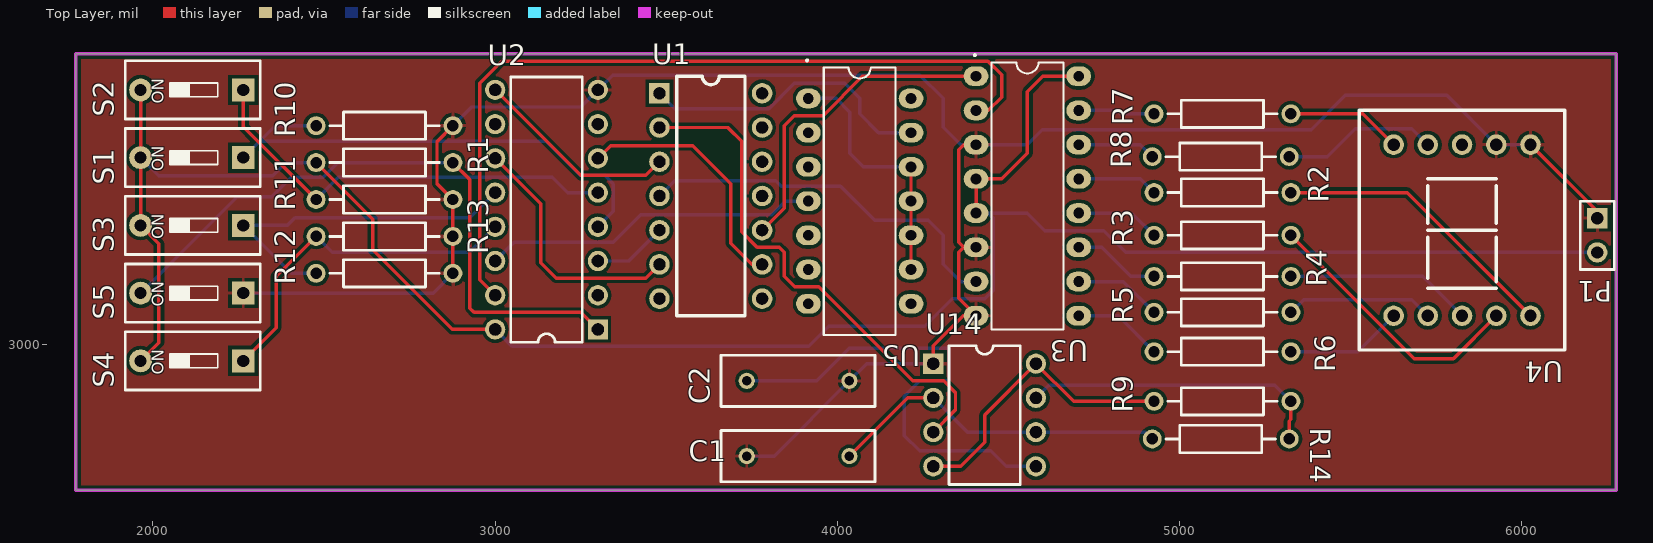
[diagram p0: Top Layer view]
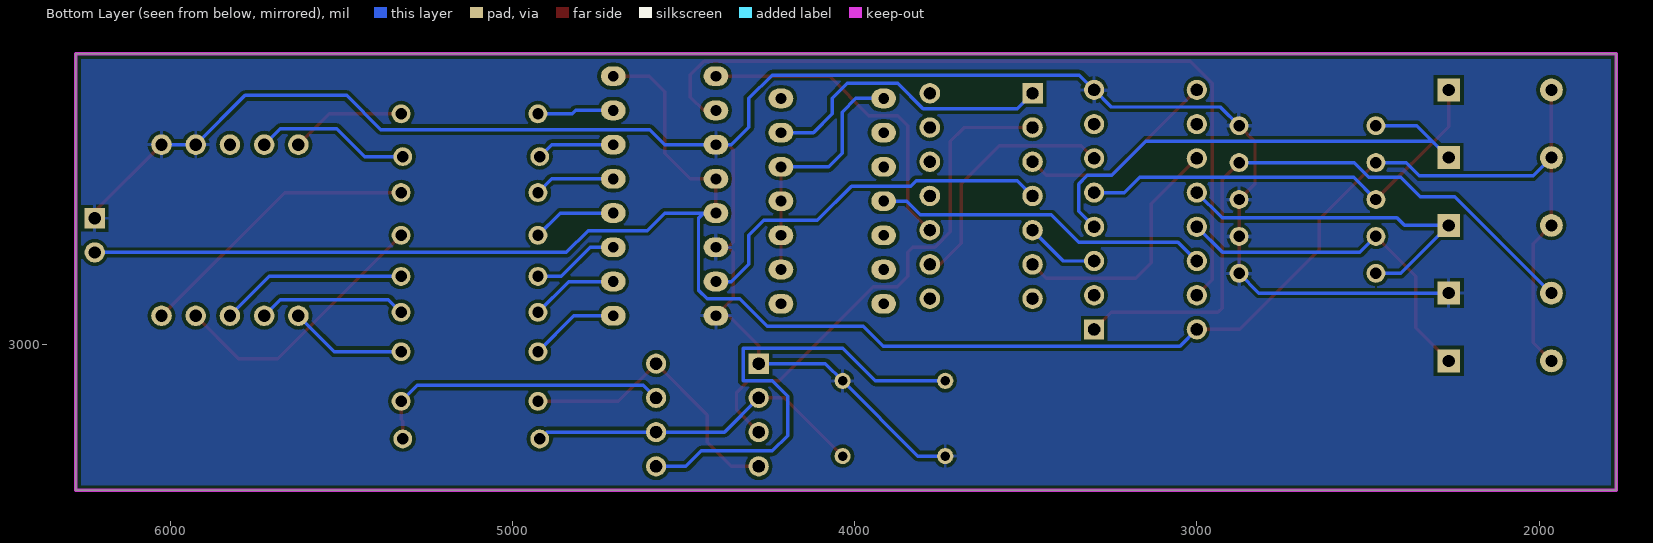
[diagram p1: Bottom Layer view, seen from below]
# Altium PCB MISC80628.PcbDoc
Units mil, origin at the board's own origin, x right, y up, seen from the top; angles counter-clockwise.
Board outline 4500 x 1275 mil, 2 copper layers (Top Layer, Bottom Layer); 28 components, 36 nets, 122 pads, 0 vias.

## Layer stack, top to bottom (the 12.6 mil dielectric is the usual default, probably not edited)
Top Solder: solder mask 0.4, Solder Resist, Dk 3.5
Top Layer: signal copper 1.4
Dielectric 1: dielectric 12.6, FR-4, Dk 4.8
Bottom Layer: signal copper 1.4
Bottom Solder: solder mask 0.4, Solder Resist, Dk 3.5

## Board outline
1775,2575 1775,3850 6275,3850 6275,2575

## Design rules (kind name [scope] priority, off if disabled: settings)
Clearance [All] p1: gap=10
PolygonConnect [All] p1: connectstyle=Relief reliefconductorwidth=10 reliefentries=4 polygonreliefangle="90 Angle" airgapwidth=10
RoutingVias [All] p1: holewidth=28 width=50 viastyle="Through Hole" minholewidth=28 minwidth=50 maxholewidth=28 maxwidth=50
SolderMaskExpansion [All] p1: expansion=4
Width [All] p1: maxlimit=10 minlimit=10 preferedwidth=10
30 further rules are at their usual default settings.

## Components (designator, comment, footprint, x,y, rotation, side; value= is the part's Value field where it differs from the comment)
C1 "Cap" RAD-0.3 3885,2675 r0 top
C2 "Cap" RAD-0.3 3885,2895 r180 top
P1 "Header 2" HDR1X2 6220,3370 r270 top
R1 "Res2" AXIAL-0.4 2676.56,3532.56 r180 top
R2 "Res2" AXIAL-0.4 5125,3445 r180 top
R3 "Res2" AXIAL-0.4 5125,3320 r180 top
R4 "Res2" AXIAL-0.4 5125,3200 r180 top
R5 "Res2" AXIAL-0.4 5125,3095 r180 top
R6 "Res2" AXIAL-0.4 5125,2980 r180 top
R7 "Res2" AXIAL-0.4 5125,3675 r180 top
R8 "Res2" AXIAL-0.4 5120,3550 r180 top
R9 "Res2" AXIAL-0.4 5125,2835 r180 top
R10 "Res2" AXIAL-0.4 2676.56,3640.43 r180 top
R11 "Res2" AXIAL-0.4 2676.56,3424.68 r180 top
R12 "Res2" AXIAL-0.4 2676.56,3208.94 r180 top
R13 "Res2" AXIAL-0.4 2676.56,3316.81 r180 top
R14 "Res2" AXIAL-0.4 5120,2725 r0 top
S1 "SW1-DIP2" DIP-1P 2113.94,3546.93 r90 top
S2 "SW1-DIP2" DIP-1P 2113.94,3744.8 r90 top
S3 "SW1-DIP2" DIP-1P 2113.94,3349.05 r90 top
S4 "SW1-DIP2" DIP-1P 2113.94,2953.31 r90 top
S5 "SW1-DIP2" DIP-1P 2113.94,3151.18 r90 top
U1 "CD4011" CD4011 3630,3435 r0 top
U2 "SN74LS175N_1" N016 3150,3395 r90 top
U3 "CD4511BCN" CD4511BCN 4555,3445.33 r270 top
U4 "Single-digit LED display (common cathode)" PCBComponent_1 5825,3335 r180 top
U5 "CD4012" DIP14 4065,3430.33 r270 top
U14 "NE555" DIP-8-NE555 4430,2795 r0 top

## Footprints (in the part's own frame and the unit in brackets; to place one, negate y for a bottom-side part, rotate by r counter-clockwise, add the part's x,y. Pads: shape width x height; smd on the part's side, far side on the other; paste and mask are expansions set on the pad)
AXIAL-0.4 [mm] "Axial Device, Thru-Hole; 2 Leads; 0.4 in Pin Spacing"
  round 1.4 hole 0.85: 1(-5.08,0) 2(5.08,0)
  silkscreen extent -4.06,-1.02 4.06,1.02
CD4011 [mil]
  rect 60x60 hole 35 slot 35.2 at 0 deg paste+0 mask+2: 1(-150,300)
  round 60 hole 35 slot 35.2 at 0 deg paste+0 mask+2: 2(-150,200) 3(-150,100) 4(-150,0) 5(-150,-100) 6(-150,-200) 7(-150,-300) 8(150,-300) 9(150,-200) 10(150,-100) 11(150,0) 12(150,100) 13(150,200) 14(150,300)
  silkscreen extent -100,-350 100,350
CD4511BCN [mm]
  oval 1.462x1.828 hole 0.8 paste+0 mask+0.051: 1(-8.628,-3.81) 2(-6.088,-3.81) 3(-3.548,-3.81) 4(-1.008,-3.81) 5(1.532,-3.81) 6(4.072,-3.81) 7(6.612,-3.81) 8(9.152,-3.81) 9(9.152,3.81) 10(6.612,3.81) 11(4.072,3.81) 12(1.532,3.81) 13(-1.008,3.81) 14(-3.548,3.81) 15(-6.088,3.81) 16(-8.628,3.81)
  silkscreen extent -10.26,-3.98 10.18,2.67
DIP14 [mm]
  oval 1.462x1.827 hole 0.8 paste+0 mask+0.051: 1(-7.358,-3.81) 2(-4.818,-3.81) 3(-2.278,-3.81) 4(0.262,-3.81) 5(2.802,-3.81) 6(5.342,-3.81) 7(7.882,-3.81) 8(7.882,3.81) 9(5.342,3.81) 10(2.802,3.81) 11(0.262,3.81) 12(-2.278,3.81) 13(-4.818,3.81) 14(-7.358,3.81)
  silkscreen extent -10.26,-3.98 10.18,2.67
DIP-1P [mm] "4.1*9.9*7mm"
  rect 1.7x1.7 hole 0.9: 1(0,-3.81)
  round 1.7 hole 0.9: 2(0,3.81)
  silkscreen extent -2.16,-5.08 2.16,4.95, body extent -2.07,-4.95 2.03,4.95, height 6.65
DIP-8-NE555 [mm]
  rect 1.5x1.5 hole 0.9 slot 0.905 at 0 deg paste+0 mask+0.051: 1(-3.81,3.81)
  round 1.5 hole 0.9 slot 0.905 at 0 deg paste+0 mask+0.051: 2(-3.81,1.27) 3(-3.81,-1.27) 4(-3.81,-3.81) 5(3.81,-3.81) 6(3.81,-1.27) 7(3.81,1.27) 8(3.81,3.81)
  silkscreen extent -2.65,-5.15 2.65,5.15
HDR1X2 [mm] "Connector; Header; 2 Position"
  rect 1.5x1.5 hole 0.9: 1(0,0)
  round 1.5 hole 0.9: 2(2.54,0)
  silkscreen extent -1.27,-1.27 3.81,1.27
N016 [mm]
  rect 1.5x1.5 hole 0.9 slot 0.905 at 90 deg paste+0 mask+0.051: 1(-8.89,-3.81)
  round 1.5 hole 0.9 slot 0.905 at 90 deg paste+0 mask+0.051: 2(-6.35,-3.81) 3(-3.81,-3.81) 4(-1.27,-3.81) 5(1.27,-3.81) 6(3.81,-3.81) 7(6.35,-3.81) 8(8.89,-3.81) 9(8.89,3.81) 10(6.35,3.81) 11(3.81,3.81) 12(1.27,3.81) 13(-1.27,3.81) 14(-3.81,3.81) 15(-6.35,3.81) 16(-8.89,3.81)
  silkscreen extent -9.85,-2.65 9.85,2.65
PCBComponent_1 [mil]
  round 60 hole 36 paste+0 mask+2: 1(-200,250) 2(-100,250) 3(0,250) 4(100,250) 5(200,250) 6(200,-250) 7(100,-250) 8(0,-250) 9(-100,-250) 10(-200,-250)
  silkscreen extent -300,-350 300,350
RAD-0.3 [mm] "Radial Cap, Thru-Hole; 2 Leads; 0.3 in Pin Spacing"
  round 1.2 hole 0.7: 1(-3.81,0) 2(3.81,0)
  silkscreen extent -5.71,-1.91 5.71,1.91

## Part data
C1 C2: "Capacitor"
P1: "Header, 2-Pin"
R1 R2 R3 R4 R5 R6 R7 R8 R9 R10 R11 R12 R13 R14: "Resistor"
U4: library part 一位数码管（共阴极）
U5: library part CD4012BM
U14: library part "NE555 (2)"

## Nets (pads, with @x,y where several pads share a name; then routed paths per layer and width w, separated by ;. In a path a pad name is that pad's centre, name@x,y a point inside that pad or via, vN(x,y) a via of type N, cw(c..) or ccw(c..) an arc to the next point about the centre after c; other vN are vias at no path point)
+5: P1.2 R1.2 S1.2 S2.2 S3.2 S4.2 U2.16 U3.4 U3.5 U3.16 | length 6431.4
  Top Layer w10: S4.2 2017,3006.37 2017,3295.99 S3.2 S1.2 S2.2 ; R1.2 2642,3367.12 2642,3278 2875,3045 U2.16 ; U3.5 U3.4 4480,3485 4555,3560 4555,3740 4600,3785 U3.16
  Bottom Layer w10: S1.2 2016.87,3494 2350,3494 2388.56,3532.56 R1.2 ; U2.16 3049,2996 3916,2996 3974,3054 4255,3054 4336,3135 4431,3135 4456,3160 4456,3370 4441,3385 ; U3.5 4441,3385 ; P1.2 4842,3270 4778,3334 4606,3334 4555,3385 4441,3385
GND: C1.1 C2.1 P1.1 R10.1 R11.1 R12.1 R13.1 S5.1 U2.8 U3.3 U3.6 U3.8 U4.9 U4.10 U14.1 | length 6346.6
  Top Layer w10: R12.1 R13.1 R11.1 2830,3471.25 2830,3593.87 R10.1 ; U14.1 4280,2997 4368,3085 U3.8 4354,3136 4354,3270 4369,3285 ; U3.6 4369,3285 ; U3.3 4369,3585 4354,3570 4354,3300 4369,3285 ; U4.10 6220,3390 P1.1
  Bottom Layer w10: S5.1 2818.8,3151.18 R12.1 ; R10.1 2931.13,3695 3250,3695 U2.8 3343,3788 4241,3788 4309,3720 4309,3636 4360,3585 U3.3 4555,3585 4599,3629 5384,3629 5484,3729 5781,3729 U4.9 U4.10 ; C1.1 3815,2675 C2.1 4085,2945 U14.1
NetC1_2: C1.2 R14.1 U14.2 U14.6 | length 1005.1
  Top Layer w10: C1.2 4205,2845 U14.2
  Bottom Layer w10: U14.2 4380,2745 U14.6 4900,2745 R14.1
NetC2_2: C2.2 U14.5 | length 1410.3
  Bottom Layer w10: C2.2 3940,2895 4035,2990 4325,2990 4325,2895 4240,2895 4195,2850 4195,2735 4240,2690 4448,2690 4493,2645 U14.5
NetR1_1: R1.1 S5.2 U2.1 | length 1916.3
  Top Layer w10: R1.1 2926,3483.12 2926,3107 2938,3095 3250,3095 U2.1
  Bottom Layer w10: S5.2 2245.76,3433 2347,3433 2404,3490 2497.44,3490 2540,3532.56 R1.1
NetR2_1: R2.1 U4.1 | length 849.1
  Top Layer w10: R2.1 5665,3445 U4.1
NetR2_2: R2.2 U3.13 | length 236.6
  Bottom Layer w10: U3.13 4885,3485 R2.2
NetR3_1: R3.1 U4.2 | length 800.9
  Top Layer w10: R3.1 5685,2960 5800,2960 U4.2
NetR3_2: R3.2 U3.12 | length 246.9
  Bottom Layer w10: U3.12 4860,3385 R3.2
NetR4_1: R4.1 U4.3 | length 547.6
  Bottom Layer w10: R4.1 5710,3200 U4.3
NetR4_2: R4.2 U3.11 | length 255.2
  Bottom Layer w10: U3.11 4772,3285 4857,3200 R4.2
NetR5_1: R5.1 U4.4 | length 434.8
  Bottom Layer w10: R5.1 5362,3132 5678,3132 U4.4
NetR5_2: R5.2 U3.10 | length 257.3
  Bottom Layer w10: U3.10 4835,3185 R5.2
NetR6_1: R6.1 U4.5 | length 343.5
  Bottom Layer w10: R6.1 5520,2980 U4.5
NetR6_2: R6.2 U3.9 | length 263.5
  Bottom Layer w10: U3.9 4820,3085 R6.2
NetR7_1: R7.1 U4.6 | length 337.3
  Top Layer w10: R7.1 5535,3675 U4.6
NetR7_2: R7.2 U3.15 | length 224.1
  Bottom Layer w10: U3.15 4815,3685 4825,3675 R7.2
NetR8_1: R8.1 U4.7 | length 458.4
  Bottom Layer w10: R8.1 5431,3550 5513,3632 5678,3632 U4.7
NetR8_2: R8.2 U3.14 | length 229.5
  Bottom Layer w10: U3.14 4885,3585 R8.2
NetR9_1: R9.1 R14.2 U14.7 | length 891.9
  Top Layer w10: R14.2 5320,2777 5325,2782 R9.1
  Bottom Layer w10: U14.7 4617,2882 5278,2882 R9.1
NetR9_2: R9.2 U14.4 U14.8 | length 861.7
  Top Layer w10: U14.4 4360,2645 4430,2715 4430,2795 U14.8 4690,2835 R9.2
NetR10_2: R10.2 S1.1 U2.4 | length 1479.8
  Bottom Layer w10: S1.1 2312.01,3595 ; R10.2 2357.44,3640.43 2312.01,3595 ; U2.4 3345,3390 3345,3470 3320,3495 3249,3495 3149,3595 2312.01,3595
NetR11_2: R11.2 S2.1 U2.5 | length 1277.3
  Top Layer w10: S2.1 2263.94,3637.31 R11.2
  Bottom Layer w10: R11.2 2541.87,3490 3167,3490 3212,3445 U2.5
NetR12_2: R12.2 S3.1 U2.12 | length 1046.5
  Bottom Layer w10: R12.2 2404.06,3208.94 S3.1 2393.06,3349.06 2415,3371 2926,3371 U2.12
NetR13_2: R13.2 S4.1 U2.13 | length 1025.5
  Top Layer w10: S4.1 2360,3049.37 2360,3200.25 R13.2
  Bottom Layer w10: R13.2 2523.37,3270 2925,3270 U2.13
NetU1_1: U1.1 U5.13 | length 870.3
  Bottom Layer w10: U1.1 3525,3690 3800,3690 3874,3764 4021,3764 4065,3720 4065,3675 4120,3620 U5.13
NetU1_2: U1.2 U14.3 | length 1524.2
  Top Layer w10: U1.2 3680,3635 3720,3595 3720,3330 3765,3285 3830,3285 3845,3270 3845,3200 3875,3170 3945,3170 4220,2895 4310,2895 4345,2860 4345,2810 U14.3
NetU1_3: U1.3 U2.9 | length 600.1
  Top Layer w10: U2.9 3250,3495 3440,3495 U1.3
NetU1_4: U1.4 U3.7 | length 1115
  Bottom Layer w10: U1.4 3525,3480 3820,3480 3836,3464 4009,3464 4109,3364 4265,3364 4309,3320 4309,3236 4360,3185 U3.7
NetU1_5: U1.5 U2.3 | length 217.3
  Bottom Layer w10: U2.3 3390,3245 U1.5
NetU1_6: U1.6 U2.11 | length 742.3
  Top Layer w10: U2.11 3133,3412 3133,3240 3178,3195 3440,3195 U1.6
NetU1_9: U1.9 U2.6 | length 741
  Top Layer w10: U2.6 3337,3582 3577,3582 3688,3471 3688,3297 3750,3235 U1.9
NetU1_10: U1.10 U3.1 | length 952.6
  Top Layer w10: U1.10 3844,3399 3844,3640 3874,3670 3958,3670 4073,3785 U3.1
NetU2_14: U2.14 U5.4 | length 987.5
  Bottom Layer w10: U2.14 3055,3300 3345,3300 3425,3380 3808,3380 3848,3420 U5.4
NetU2_15: U2.15 U3.2 | length 2362.9
  Top Layer w10: U2.15 2955,3190 2955,3765 3019,3829 4440,3829 4480,3789 4480,3724 4441,3685 U3.2
NetU5_1: U5.1 U5.9 U5.10 U5.11 U5.12 | length 753.1
  Top Layer w10: U5.9 U5.10 U5.11 U5.12
  Bottom Layer w10: U5.1 3996,3720 4036,3680 4036,3560 4076,3520 U5.12
pads on no net: U1.7 U1.8 U1.11 U1.12 U1.13 U1.14 U2.2 U2.7 U2.10 U4.8 U5.2 U5.3 U5.5 U5.6 U5.7 U5.8 U5.14

## Polygon pours and split planes (outlines as drawn)
GND on Top Layer "Top Layer-No Net" (solid, remove dead copper, pour order 0): 1710,4040 1800,3950 6510,3950 6510,2505 6420,2415 6400,2395 1605,2395
GND on Bottom Layer "Top Layer-No Net" (solid, remove dead copper, pour order 2): 1575,4105 6340,4105 6510,3935 6450,3875 6450,1950 1565,1950 1420,2095

## Keep-outs
Keep-Out Layer:
  lines w10: 1775,2575 1775,3850 1800,3850 6275,3850 6275,2607.07 6275,2575 6265,2575 6235,2575 1775,2575